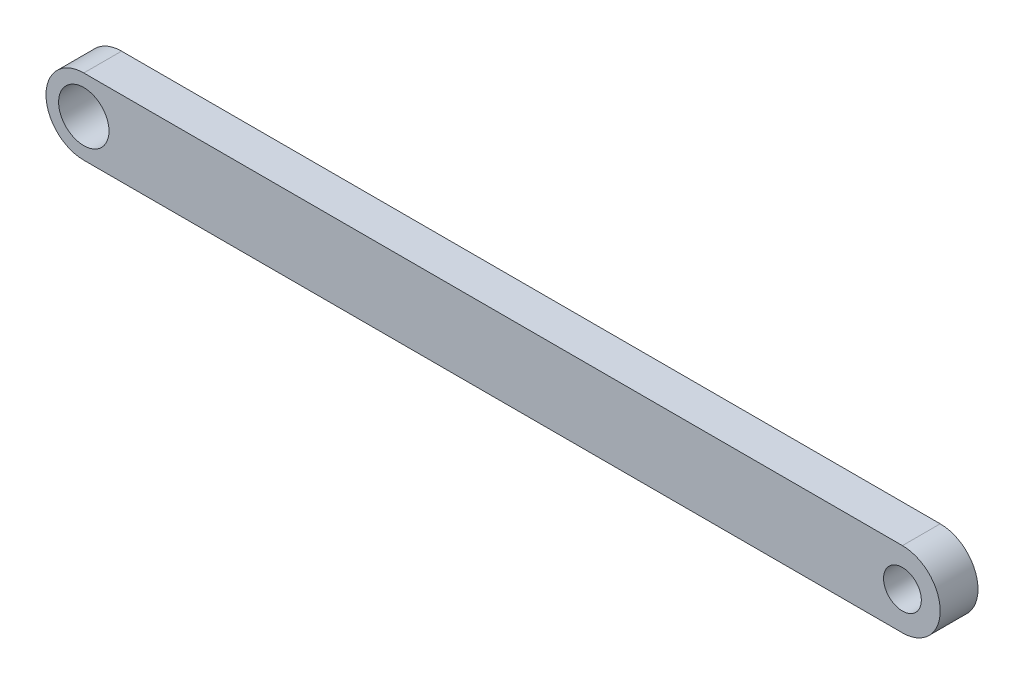
from build123d import *

# Parameters (mm, degrees)
SKETCH1_R           = 4
SKETCH1_R_2         = 3
BOSS_EXTRUDE1_DEPTH = 6
SCALE1_SCALE        = 0.5


with BuildPart() as part:
    # Sketch1 → Boss-Extrude1 (new body)
    with BuildSketch(Plane.XY):
        with BuildLine():
            Line((-32.375641401, 3), (97.624358599, 3))
            ThreePointArc((97.624358599, 3), (103.624358599, -3), (97.624358599, -9))
            Line((97.624358599, -9), (-32.375641401, -9))
            ThreePointArc((-32.375641401, -9), (-38.375641401, -3), (-32.375641401, 3))
        make_face()
        with Locations((-32.375641401, -3)):
            Circle(SKETCH1_R, mode=Mode.SUBTRACT)
        with Locations((97.624358599, -3)):
            Circle(SKETCH1_R_2, mode=Mode.SUBTRACT)
    extrude(amount=BOSS_EXTRUDE1_DEPTH)


with BuildPart() as part_1:
    # Scale1: scaled about (0, 0, 0)
    add(part.part.scale(SCALE1_SCALE))


solid = part_1.part
